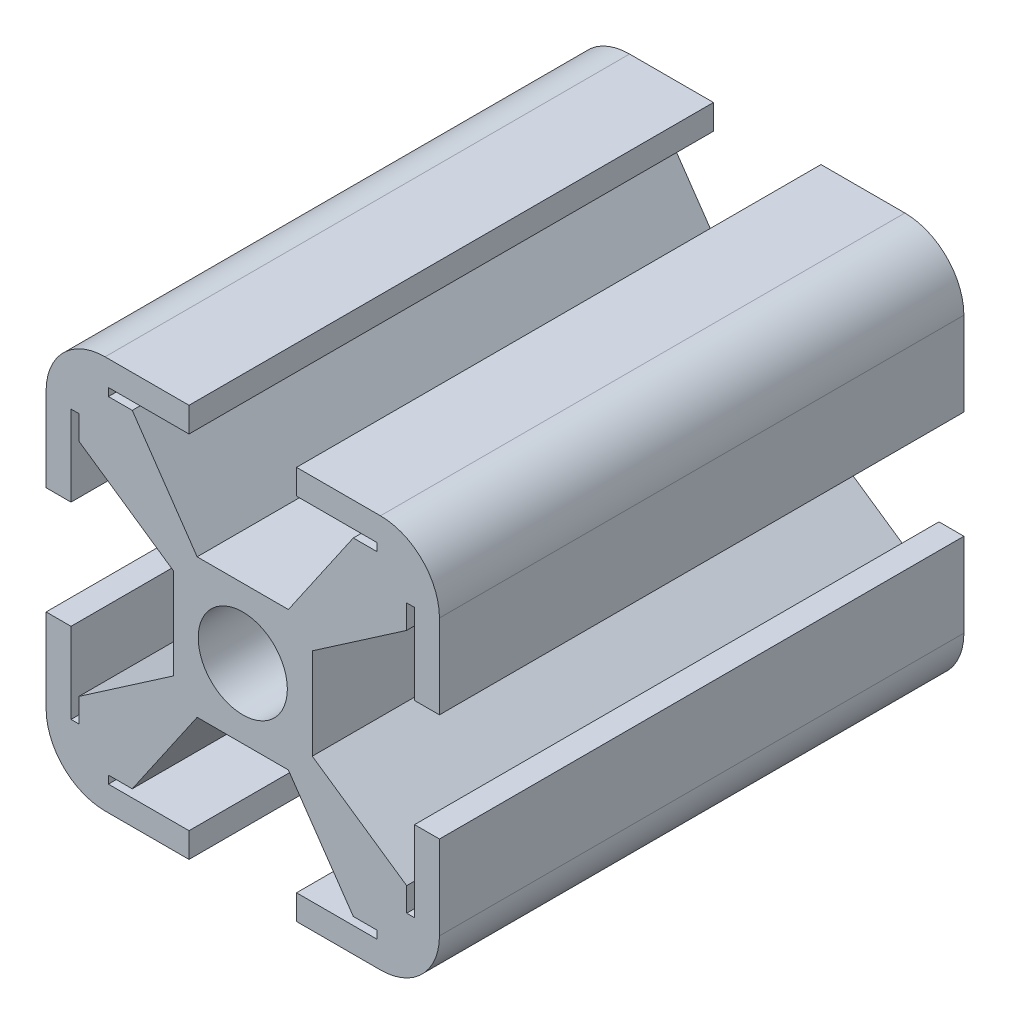
SolidWorks part; units mm, degrees
ref_plane "前视基准面" through (0, 0, 0) normal (0, 0, 1) x (1, 0, 0)
ref_plane "上视基准面" through (0, 0, 0) normal (0, 1, 0) x (1, 0, 0)
ref_plane "右视基准面" through (0, 0, 0) normal (1, 0, 0) x (0, 0, -1)
sketch "草图1" plane through (0, 0, 0) normal (0, 0, 1) x (1, 0, 0)
  line L1 (15, -15) -> (-15, -15)
  line L2 (15, -15) -> (15, 15)
  line L3 (15, 15) -> (-15, 15)
  line L4 (-15, -15) -> (-15, 15)
  line L5 (15, -15) -> (-15, 15) construction
  line L6 (15, 15) -> (-15, -15) construction
  point P0 (0, 0)
  dimension "D1" = 30
extrude "凸台-拉伸1" add sketch "草图1" along normal mid plane 40
fillet "圆角1" radius 4.5 4 edges at (15, -15, 0) (15, 15, 0) (-15, 15, 0) (-15, -15, 0)
sketch "草图2" plane through (0, 0, 20) normal (0, 0, 1) x (1, 0, 0)
  line L0 (10.5, 15) -> (-10.5, 15) construction
  line L1 (4.1, 17.2) -> (-4.1, 17.2)
  line L2 (4.1, 17.2) -> (4.1, 12.8)
  line L3 (4.1, 12.8) -> (-4.1, 12.8)
  line L4 (-4.1, 17.2) -> (-4.1, 12.8)
  line L5 (4.1, 17.2) -> (-4.1, 12.8) construction
  line L6 (4.1, 12.8) -> (-4.1, 17.2) construction
  line L7 (-10.25, 12.5) -> (-5.3, 5.3)
  line L8 (10.25, 13.1) -> (-10.25, 13.1)
  line L9 (10.25, 13.1) -> (10.25, 12.5)
  line L10 (10.25, 12.5) -> (-10.25, 12.5)
  line L11 (-10.25, 13.1) -> (-10.25, 12.5)
  line L12 (10.25, 13.1) -> (-10.25, 12.5) construction
  line L13 (10.25, 12.5) -> (-10.25, 13.1) construction
  line L14 (5.3, -5.3) -> (-5.3, -5.3)
  line L15 (5.3, -5.3) -> (5.3, 5.3)
  line L16 (5.3, 5.3) -> (-5.3, 5.3)
  line L17 (-5.3, -5.3) -> (-5.3, 5.3)
  line L18 (5.3, -5.3) -> (-5.3, 5.3) construction
  line L19 (5.3, 5.3) -> (-5.3, -5.3) construction
  line L20 (-8.4297, 12.5) -> (-3.4797, 5.3)
  line L21 (10.25, 12.5) -> (5.3, 5.3)
  line L22 (8.4297, 12.5) -> (3.4797, 5.3)
  circle A0 centre (0, 0) radius 3.4
  point P0 (0, 15)
  point P7 (0, 12.8)
  point P12 (0, 0)
  line M7 (10.5, 15) -> (-10.5, 15)
  dimension "D6" = 6.8
  dimension "D1" = 8.2
  dimension "D2" = 20.5
  dimension "D3" = 10.6
  dimension "D4" = 1.5
  dimension "D5" = 1.5
  dimension "D7" = 1.9
  dimension "D8" = 12.5
extrude "切除-拉伸1" cut sketch "草图2" against normal through all contours L2 L8 L4 L3 | L8 L2 L4 M7 | L8 L11 L10 L9 L2 L3 L4 | L22 L10 L20 L16 | A0
pattern_circular "阵列(圆周)1" count 4 over 360 about axis through (0, 0, 0) along (0, 0, 1) of "切除-拉伸1"
